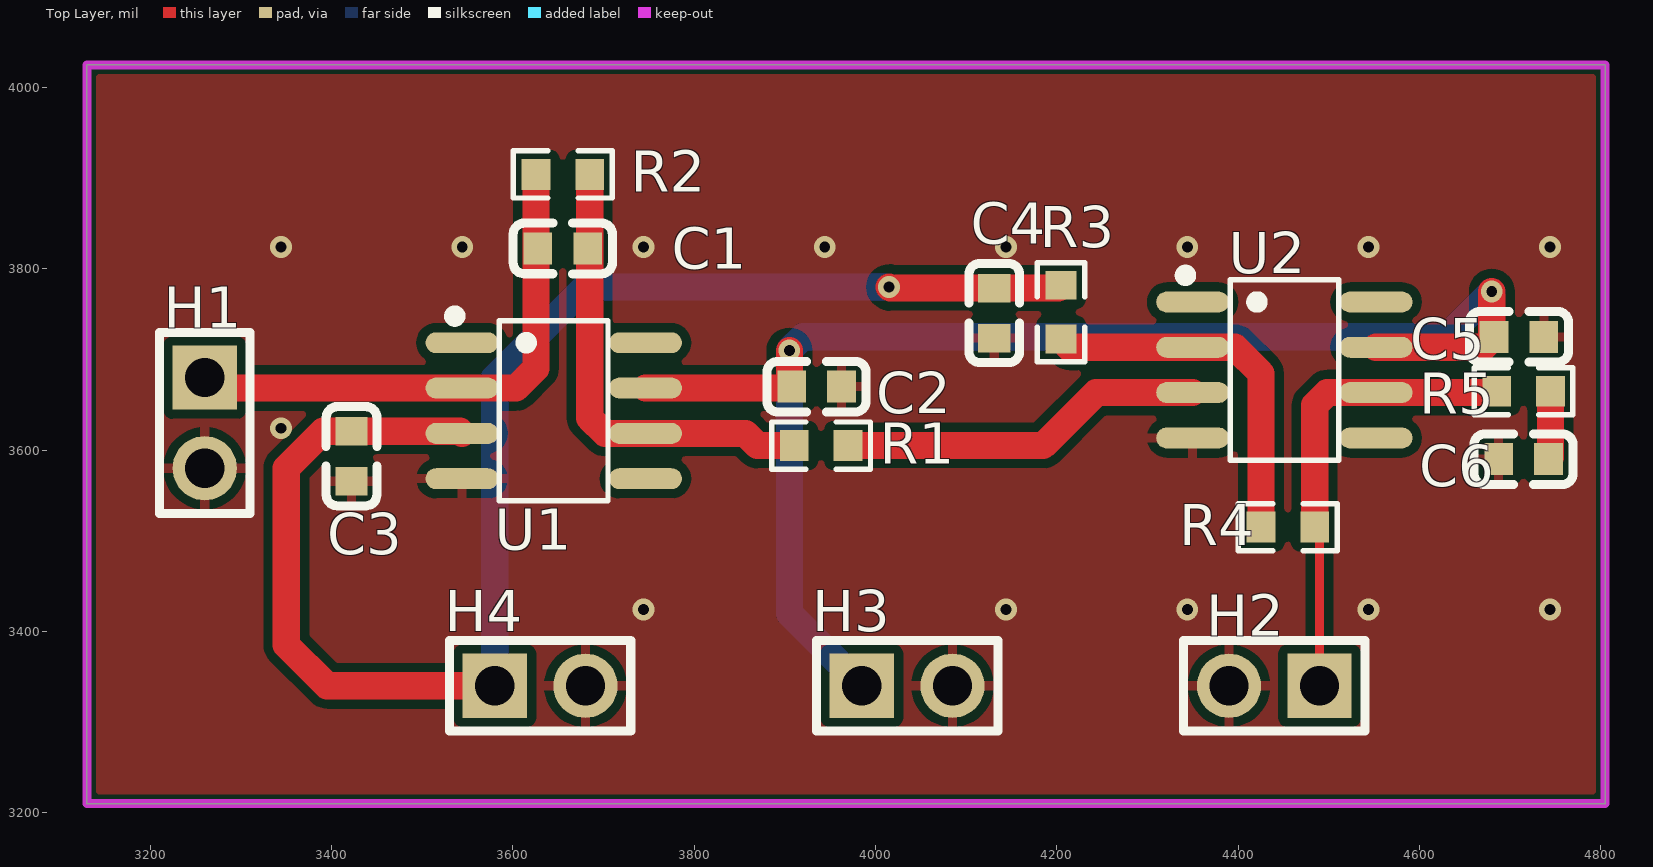
[diagram p0: Top Layer view]
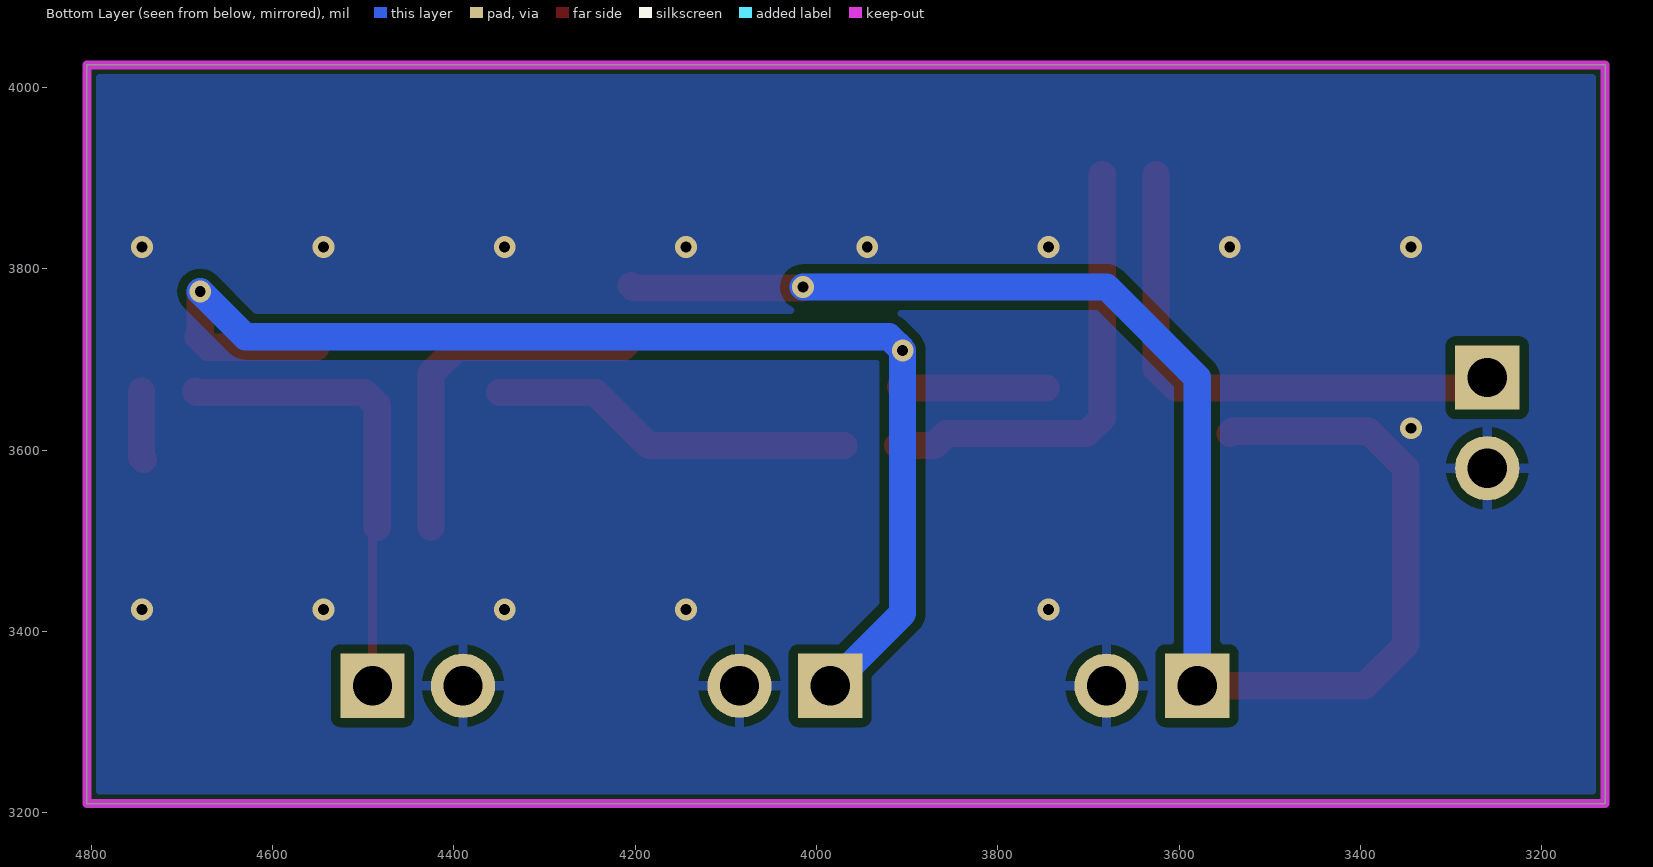
[diagram p1: Bottom Layer view, seen from below]
# Altium PCB MISC51758.pcbdoc
Units mil, origin at the board's own origin, x right, y up, seen from the top; angles counter-clockwise.
Board outline 1675 x 815 mil, 2 copper layers (Top Layer, Bottom Layer), stack 62.206 mil thick; 17 components, 9 nets, 46 pads, 17 vias.

## Layer stack, top to bottom
Top Solder Mask Layer: solder mask 0.394, Dk 3.3
Top Layer: signal copper 1.379
Dielectric1: surface 59.449, FR4, Dk 4.5
Bottom Layer: signal copper 1.378
Bottom Solder Mask Layer: solder mask 0.394, Dk 3.3

## Board outline
3130,4025 3130,3210 4805,3210 4805,4025

## Design rules (kind name [scope] priority, off if disabled: settings)
BoardOutlineClearance copperThickness2oz_1 [All] p2 off: genericclearance=7.99 ignorepadtopadclearanceinfootprint=FALSE except(0: Arc-SplitContinuation Track-SplitContinuation SMDPad-SplitContinuation THPad-SplitContinuation Via-SplitContinuation Fill-SplitContinuation Region-SplitContinuation Poly-SplitContinuation Text-SplitContinuation Hole-SplitContinuation; 5.98: Arc-CutoutEdge SMDPad-CutoutEdge THPad-CutoutEdge Via-CutoutEdge Fill-CutoutEdge Region-CutoutEdge Text-CutoutEdge; 6.93: Hole-OutlineEdge Hole-CutoutEdge; 10: Poly-OutlineEdge Poly-CutoutEdge; 11.81: Arc-OutlineEdge Track-OutlineEdge SMDPad-OutlineEdge THPad-OutlineEdge Via-OutlineEdge Fill-OutlineEdge Region-OutlineEdge Text-OutlineEdge Track-CutoutEdge)
BoardOutlineClearance copperThickness1oz_1 [All] p4: genericclearance=4.02 ignorepadtopadclearanceinfootprint=FALSE except(0: Arc-SplitContinuation Track-SplitContinuation SMDPad-SplitContinuation THPad-SplitContinuation Via-SplitContinuation Fill-SplitContinuation Region-SplitContinuation Poly-SplitContinuation Text-SplitContinuation Hole-SplitContinuation; 6: SMDPad-CutoutEdge THPad-CutoutEdge Via-CutoutEdge Fill-CutoutEdge Region-CutoutEdge Text-CutoutEdge; 6.93: Hole-OutlineEdge Hole-CutoutEdge; 10: Poly-OutlineEdge Poly-CutoutEdge; 11.8: Arc-OutlineEdge Track-OutlineEdge SMDPad-OutlineEdge THPad-OutlineEdge Via-OutlineEdge Fill-OutlineEdge Region-OutlineEdge Text-OutlineEdge; 11.81: Arc-CutoutEdge Track-CutoutEdge)
Clearance copperThickness2oz [All] p1 off: gap=7.99 ignorepadtopadclearanceinfootprint=FALSE except(5.98: SMDPad-Track SMDPad-SMDPad THPad-Track SMDPad-THPad THPad-THPad Track-Via SMDPad-Via THPad-Via Via-Via Fill-Track Region-Track Fill-SMDPad Region-SMDPad Fill-THPad Region-THPad Fill-Via Region-Via Fill-Fill Fill-Region Region-Region Arc-Track Arc-SMDPad Arc-THPad Arc-Via Fill-Arc Region-Arc Arc-Arc Text-Track SMDPad-Text Text-THPad Text-Via Fill-Text Region-Text Arc-Text Text-Text; 6.93: Hole-Track Hole-SMDPad Hole-THPad Hole-Via Fill-Hole Region-Hole Hole-Arc Hole-Text; 10: Poly-Track Poly-SMDPad Poly-THPad Poly-Via Poly-Fill Poly-Region Poly-Poly Poly-Arc Poly-Text Poly-Hole)
Clearance copperThickness1oz [All] p3: gap=4.02 ignorepadtopadclearanceinfootprint=FALSE except(5.98: SMDPad-Track SMDPad-SMDPad THPad-Track SMDPad-THPad THPad-THPad Track-Via SMDPad-Via THPad-Via Via-Via Fill-Track Region-Track Fill-SMDPad Region-SMDPad Fill-THPad Region-THPad Fill-Via Region-Via Fill-Fill Fill-Region Region-Region; 6: Arc-Track Arc-SMDPad Arc-THPad Arc-Via Fill-Arc Region-Arc Arc-Arc Text-Track SMDPad-Text Text-THPad Text-Via Fill-Text Region-Text Arc-Text Text-Text; 6.93: Hole-Track Hole-SMDPad Hole-THPad Hole-Via Fill-Hole Region-Hole Hole-Arc Hole-Text; 10: Poly-Track Poly-SMDPad Poly-THPad Poly-Via Poly-Fill Poly-Region Poly-Poly Poly-Arc Poly-Text Poly-Hole)
Creepage creepage [All] p1: checkdistance=0 ignoreinternallayers=TRUE applytopolygonpour=TRUE
DiffPairsRouting differentialPair [All] p1: maxlimit=6 minlimit=6 mostfreqgap=6 toplayer_minwidth=5 toplayer_prefwidth=10 toplayer_maxwidth=100 toplayer_mingap=6 toplayer_prefgap=6 toplayer_maxgap=6 bottomlayer_minwidth=5 bottomlayer_prefwidth=10 bottomlayer_maxwidth=100 bottomlayer_mingap=6 bottomlayer_prefgap=6 bottomlayer_maxgap=6 maxuncoupledlength=10
HoleToHoleClearance otherClearance [All] p1: gap=11.81 allowstackedmicrovias=TRUE
Length netLength [All] p1: minlimit=0 maxlimit=0
MatchedLengths netLengthTolerance [All] p1: tolerance=1000
PasteMaskExpansion pasteMaskExpansion [All] p1: expansion=0
PlaneConnect innerPlane [All] p1: planeconnectstyle=Relief reliefexpansion=20 reliefentries=4 reliefconductorwidth=10 reliefairgap=10
PolygonConnect copperRegion [(InNet('GND'))] p1: connectstyle=Relief reliefconductorwidth=10 reliefentries=4 polygonreliefangle="90 Angle" airgapwidth=10 via.connectstyle=Relief via.reliefconductorwidth=10 via.reliefentries=4 via.polygonreliefangle="90 Angle" via.airgapwidth=10
RoutingVias viaSize [All] p1: holewidth=12.01 width=24.02 viastyle="Through Hole" minholewidth=11.81 minwidth=19.68 maxholewidth=248.03 maxwidth=393.7
SolderMaskExpansion solderMaskExpansion [IsVia] p1: expansion=-1000 istentingtop=TRUE
SolderMaskExpansion solderMaskExpansion [All] p2: expansion=2 istentingtop=FALSE
Width copperThickness2oz_2 [All] p1 off: maxlimit=100 minlimit=8 preferedwidth=10
Width copperThickness1oz_2 [All] p2: maxlimit=100 minlimit=5 preferedwidth=10

## Components (designator, comment, footprint, x,y, rotation, side; value= is the part's Value field where it differs from the comment)
C1 "10nF" C0603 3655.02,3822.49 r0 top
C2 "100nF" C0603 3935,3670 r180 top
C3 "100nF" C0603 3421.97,3593.24 r90 top
C4 "100nF" C0603 4131.07,3751.22 r90 top
C5 "100nF" C0603 4710,3725 r180 top
C6 "100nF" C0603 4715,3590 r180 top
H1 "" HDR-TH_2P-P2.54-V-M-1 3260,3630 r270 top
H2 "" HDR-TH_2P-P2.54-V-M-1 4440,3340 r180 top
H3 "" HDR-TH_2P-P2.54-V-M-1 4035,3340 r0 top
H4 "" HDR-TH_2P-P2.54-V-M-1 3630,3340 r0 top
R1 "10K" R0603 3940,3605 r0 top
R2 "1. 1MEG" R0603 3655.02,3904.14 r0 top
R3 "8.2K" R0603 4204.67,3752.12 r270 top
R4 "120K" R0603 4455,3515 r0 top
R5 "5.1K" R0603 4715,3665 r0 top
U1 "OPA445AUG4" SOIC-8_L4.9-W3.9-P1.27-LS6.0-BL 3645.02,3643.45 r270 top
U2 "OPA445AUG4" SOIC-8_L4.9-W3.9-P1.27-LS6.0-BL 4451.14,3688.45 r270 top

## Footprints (in the part's own frame and the unit in brackets; to place one, negate y for a bottom-side part, rotate by r counter-clockwise, add the part's x,y. Pads: shape width x height; smd on the part's side, far side on the other; paste and mask are expansions set on the pad)
C0603 [mm]
  rect 0.8x0.9 smd: 1(-0.7,0) 2(0.7,0)
  silkscreen extent -1.39,-0.71 1.39,0.71
HDR-TH_2P-P2.54-V-M-1 [mm]
  rect 1.8x1.8 hole 1.1: 1(-1.27,0)
  round 1.8 hole 1.1: 2(1.27,0)
  silkscreen extent -2.54,-1.27 2.54,1.27
R0603 [mil]
  rect 31.75x34.02 smd paste-3937.01 mask+2: 1(-29.66,0) 2(29.66,0)
  silkscreen extent -55,-26 55,26
SOIC-8_L4.9-W3.9-P1.27-LS6.0-BL [mm]
  oval 0.588x2.045 smd: 1(-1.905,-2.57) 2(-0.635,-2.57) 3(0.635,-2.57) 4(1.905,-2.57) 5(1.905,2.57) 6(0.635,2.57) 7(-0.635,2.57) 8(-1.905,2.57)
  silkscreen extent -2.8,-2.92 2.53,1.52

## Via types
v1: diameter 24.02, hole 12, Top Layer to Bottom Layer, 17 vias

## Nets (pads, with @x,y where several pads share a name; then routed paths per layer and width w, separated by ;. In a path a pad name is that pad's centre, name@x,y a point inside that pad or via, vN(x,y) a via of type N, cw(c..) or ccw(c..) an arc to the next point about the centre after c; other vN are vias at no path point)
1V: C3.2 C4.2 H4.1 R3.1 U1.3 | length 1663.2
  Top Layer w30: U1.3 3541.49,3620.8 C3.2 3390.8,3620.8 3350,3580 3350,3385 3395,3340 H4.1 ; v1(4015,3780) 4016.22,3778.78 C4.2 4201.67,3778.78 R3.1
  Bottom Layer w30: H4.1 3580,3680 3680,3780 v1(4015,3780)
3V3: C2.2 C5.2 H3.1 U1.7 U2.7 | length 1593.9
  Top Layer w30: U1.7 3905.89,3668.45 C2.2 3905,3672.44 v1(3905,3710) ; U2.7 4670.89,3713.45 C5.2 4680,3727.44 v1(4680,3775)
  Bottom Layer w30: H3.1 3905,3420 v1(3905,3710) 3920,3725 4630,3725 v1(4680,3775)
$1N1: C1.2 R1.1 R2.2 U1.6 | length 507
  Top Layer w30: R2.2 3684.68,3635.32 3701.55,3618.45 U1.6 3856.55,3618.45 3870,3605 R1.1
$1N2: C1.1 H1.1 R2.1 U1.2 | length 593
  Top Layer w30: H1.1 3271.55,3668.45 U1.2 3603.45,3668.45 3625.36,3690.36 R2.1
$1N9: R1.2 U2.3 | length 404.5
  Top Layer w30: R1.2 4185,3605 4243.45,3663.45 U2.3
$1N16: H2.1 R4.2 R5.1 U2.6 | length 518.9
  Top Layer w10: R4.2 4490,3509.66 H2.1
  Top Layer w30: R4.2 4484.66,3649.66 4498.45,3663.45 U2.6 4683.79,3663.45 R5.1
$1N17: R3.2 R4.1 U2.2 | length 406
  Top Layer w30: R3.2 4213.67,3713.45 U2.2 4396.55,3713.45 4425.34,3684.66 R4.1
$1N18: C6.1 R5.2 | length 75.9
  Top Layer w30: C6.1 4744.66,3592.1 R5.2
GND: C2.1 C3.1 C4.1 C5.1 C6.2 H1.2 H2.2 H3.2 H4.2 U1.4 U2.4
  other v1: 3744.1,3424.1 4144.1,3424.1 4344.1,3424.1 4544.1,3424.1 4744.1,3424.1 3344.1,3624.1 3344.1,3824.1 3544.1,3824.1 3744.1,3824.1 3944.1,3824.1 4144.1,3824.1 4344.1,3824.1 4544.1,3824.1 4744.1,3824.1
pads on no net: U1.1 U1.5 U1.8 U2.1 U2.5 U2.8

## Polygon pours and split planes (outlines as drawn)
GND on Top Layer (solid, remove dead copper, pour order 0): 3000,4125 3000,3045 4930,3045 4930,4125
GND on Bottom Layer (solid, remove dead copper, pour order 2): 3070,4095 3070,3000 4960,3000 4960,4095

## Keep-outs
Board Outline Layer:
  the board outline again, w10